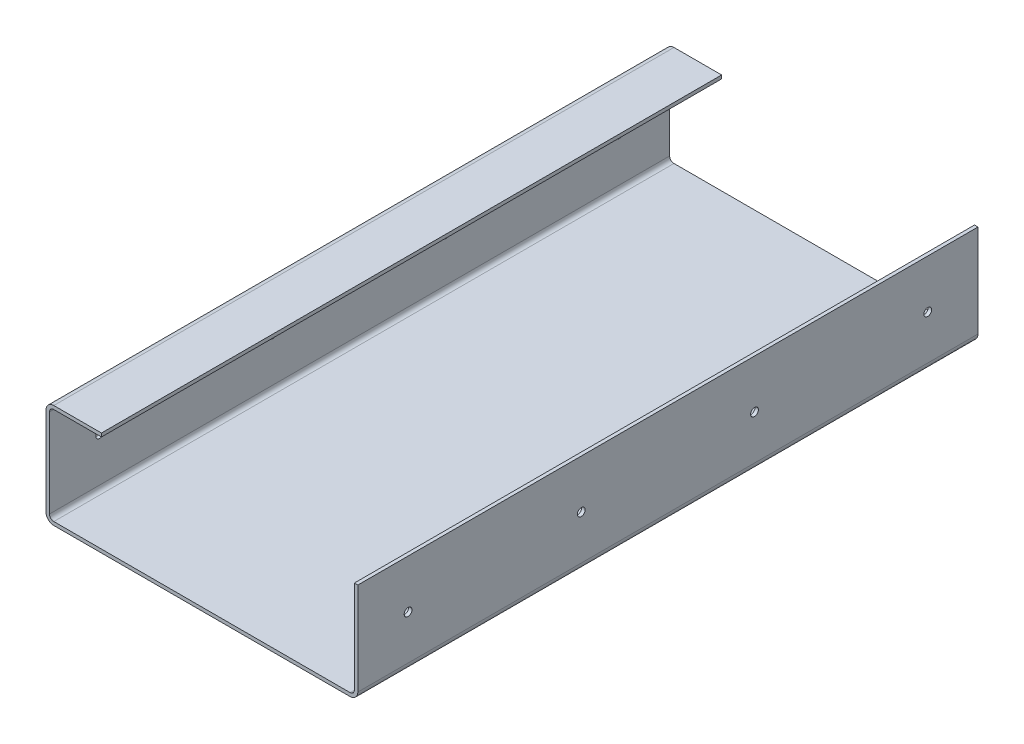
SolidWorks part; units mm, degrees
material "1023 碳钢板 (SS)"
ref_plane "Front Plane" through (0, 0, 0) normal (0, 0, 1) x (1, 0, 0)
ref_plane "Top Plane" through (0, 0, 0) normal (0, 1, 0) x (1, 0, 0)
ref_plane "Right Plane" through (0, 0, 0) normal (1, 0, 0) x (0, 0, -1)
sketch "Sketch1" plane through (0, 0, 0) normal (0, 0, 1) x (1, 0, 0)
  line L0 (0, 0) -> (-55, 0)
  line L1 (-64, -9) -> (-64, -111)
  line L2 (-55, -120) -> (287, -120)
  line L3 (296, -111) -> (296, -4)
  line L4 (0, -4) -> (-55, -4)
  line L5 (-60, -9) -> (-60, -111)
  line L6 (-55, -116) -> (287, -116)
  line L7 (292, -111) -> (292, -4)
  line L8 (0, 0) -> (0, -4)
  line L9 (296, -4) -> (292, -4)
  arc A0 (287, -120) -> (296, -111) centre (287, -111) ccw
  arc A1 (-55, 0) -> (-64, -9) centre (-55, -9) ccw
  arc A2 (-64, -111) -> (-55, -120) centre (-55, -111) ccw
  arc A3 (-55, -4) -> (-60, -9) centre (-55, -9) ccw
  arc A4 (-60, -111) -> (-55, -116) centre (-55, -111) ccw
  arc A5 (287, -116) -> (292, -111) centre (287, -111) ccw
  point P8 (296, -120)
  point P11 (-64, 0)
  point P14 (-64, -120)
  dimension "D5" = 9
  dimension "D1" = 64
  dimension "D2" = 120
  dimension "D3" = 116
  dimension "D4" = 360
  dimension "D6" = 4
extrude "Boss-Extrude1" add sketch "Sketch1" along normal blind 716 contours L9 L7 A5 L6 A4 L5 A3 L4 L8 L0 A1 L1 A2 L2 A0 L3
sketch "Sketch2" plane through (-64, 0, 0) normal (-1, 0, 0) x (0, 0, 1)
  line L0 (0, -9) -> (0, -111) construction
  circle A0 centre (58, -60) radius 4.5
  circle A1 centre (258, -60) radius 4.5
  circle A2 centre (458, -60) radius 4.5
  circle A3 centre (658, -60) radius 4.5
  point P11 (0, -60)
  dimension "D5" = 9
  dimension "D1" = 200
  dimension "D2" = 200
  dimension "D3" = 58
  dimension "D4" = 200
extrude "Cut-Extrude1" cut sketch "Sketch2" against normal blind 716
